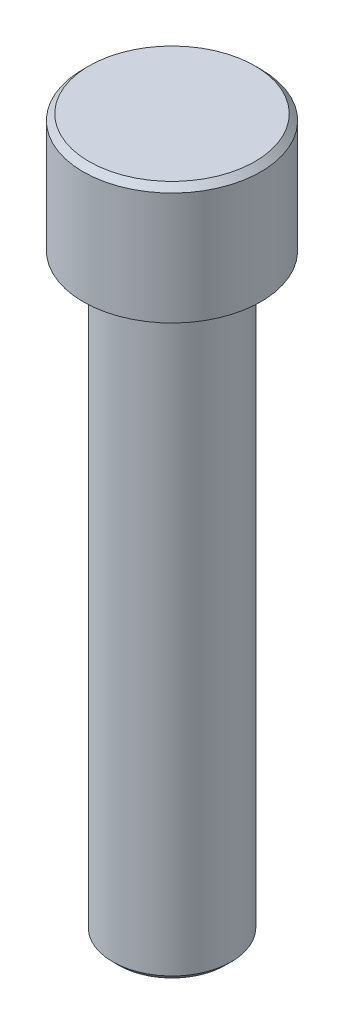
SolidWorks part; units mm, degrees
ref_plane "前视基准面" through (0, 0, 0) normal (0, 0, 1) x (1, 0, 0)
ref_plane "上视基准面" through (0, 0, 0) normal (0, 1, 0) x (1, 0, 0)
ref_plane "右视基准面" through (0, 0, 0) normal (1, 0, 0) x (0, 0, -1)
other "Configuration Table"
sketch "草图1" plane through (0, 0, 0) normal (0, 1, 0) x (1, 0, 0)
  circle A0 centre (0, 0) radius 5
  dimension "D1" = 10
extrude "凸台-拉伸1" add sketch "草图1" along normal mid plane 50 contours A0
sketch "草图2" plane through (0, 25, 0) normal (0, 1, 0) x (1, 0, 0)
  circle A0 centre (0, 0) radius 7.5
  dimension "D1" = 15
extrude "凸台-拉伸2" add sketch "草图2" along normal blind 10 contours A0
chamfer "倒角1" distance 0.5 angle 45 2 edges at (0, 35, 7.5) (0, -25, 5)
